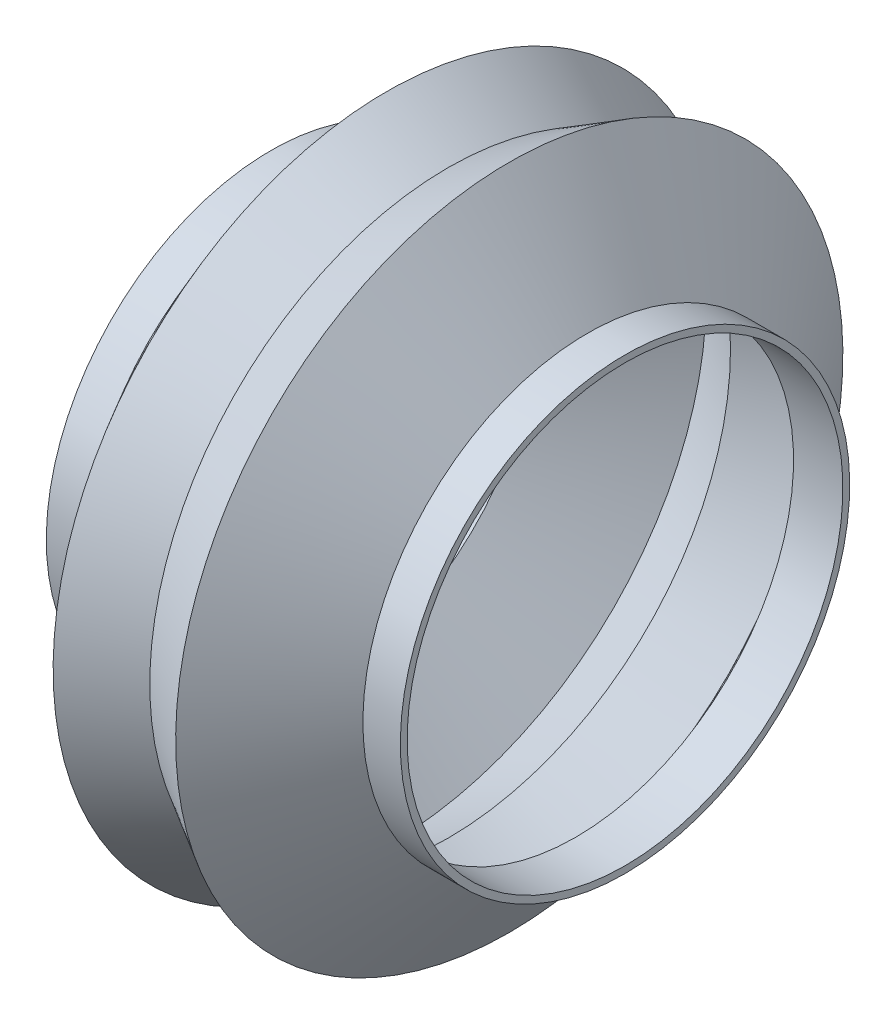
SolidWorks part; units mm, degrees
ref_plane "Front Plane" through (0, 0, 0) normal (0, 0, 1) x (1, 0, 0)
ref_plane "Top Plane" through (0, 0, 0) normal (0, 1, 0) x (1, 0, 0)
ref_plane "Right Plane" through (0, 0, 0) normal (1, 0, 0) x (0, 0, -1)
other "Configuration Table"
sketch "Sketch1" plane through (0, 0, 0) normal (0, 0, 1) x (1, 0, 0)
  line L0 (0, 31.0172) -> (0, 0) construction
  line L1 (-38.0977, 0) -> (38.0977, 0) construction
  line L2 (0, 21.9019) -> (4.5, 24.5)
  line L3 (4.5, 24.5) -> (10.25, 16.5)
  line L4 (10.25, 16.5) -> (13, 16.5)
  line L5 (13, 16.5) -> (13, 0)
  line L6 (13, 0) -> (-13, 0)
  line L7 (0, 0) -> (0, 21.9019) construction
  line L8 (-13, 16.5) -> (-13, 0)
  line L9 (-10.25, 16.5) -> (-13, 16.5)
  line L10 (-4.5, 24.5) -> (-10.25, 16.5)
  line L11 (0, 21.9019) -> (-4.5, 24.5)
  dimension "D1" = 49
  dimension "D2" = 33
  dimension "D3" = 9
  dimension "D4" = 20.5
  dimension "D5" = 26
  dimension "D6" = 120
revolve "Revolve1" add sketch "Sketch1" angle 360 about L1
sketch "Sketch2" plane through (13, 0, 0) normal (1, 0, 0) x (0, 0, -1)
  circle A0 centre (0, 0) radius 16
  dimension "D1" = 32
sketch "Sketch3" plane through (0, 0, 0) normal (0, 0, 1) x (1, 0, 0)
  line L0 (4.2162, 23.1814) -> (0, 20.7472)
  line L1 (0, 20.7472) -> (-4.2162, 23.1814)
  line L2 (-4.2162, 23.1814) -> (-9.7372, 15.5)
  line L3 (-9.7372, 15.5) -> (-12, 15.5)
  line L4 (-12, 15.5) -> (-12, 1)
  line L6 (12, 1) -> (12, 15.5)
  line L7 (12, 15.5) -> (9.7372, 15.5)
  line L8 (9.7372, 15.5) -> (4.2162, 23.1814)
  line L9 (4.5, 24.5) -> (0, 21.9019)
  line L10 (10.25, 16.5) -> (4.5, 24.5)
  line L11 (13, 16.5) -> (10.25, 16.5)
  line L12 (13, 0) -> (13, 16.5)
  line L13 (-13, 0) -> (13, 0)
  line L14 (-13, 16.5) -> (-13, 0)
  line L15 (-10.25, 16.5) -> (-13, 16.5)
  line L16 (-4.5, 24.5) -> (-10.25, 16.5)
  line L17 (0, 21.9019) -> (-4.5, 24.5)
  line L18 (4.5, 24.5) -> (0, 21.9019) construction
  line L19 (10.25, 16.5) -> (4.5, 24.5) construction
  line L20 (13, 16.5) -> (10.25, 16.5) construction
  line L21 (13, 0) -> (13, 16.5) construction
  line L22 (-13, 0) -> (13, 0) construction
  line L23 (-13, 16.5) -> (-13, 0) construction
  line L24 (-10.25, 16.5) -> (-13, 16.5) construction
  line L25 (-4.5, 24.5) -> (-10.25, 16.5) construction
  line L26 (0, 21.9019) -> (-4.5, 24.5) construction
  line L27 (-12, 1) -> (12, 1) construction
  line L28 (12, 1) -> (12, 0)
  line L29 (12, 0) -> (-12, 0)
  line L30 (-12, 0) -> (-12, 1)
  dimension "D1" = 0
  dimension "D2" = 1
revolve "Cut-Revolve1" cut sketch "Sketch3" angle 360 about L29
sketch "Sketch4" plane through (13, 0, 0) normal (1, 0, 0) x (0, 0, -1)
  circle A0 centre (0, 0) radius 16
  dimension "D1" = 32
extrude "Cut-Extrude2" cut sketch "Sketch4" against normal blind 120
